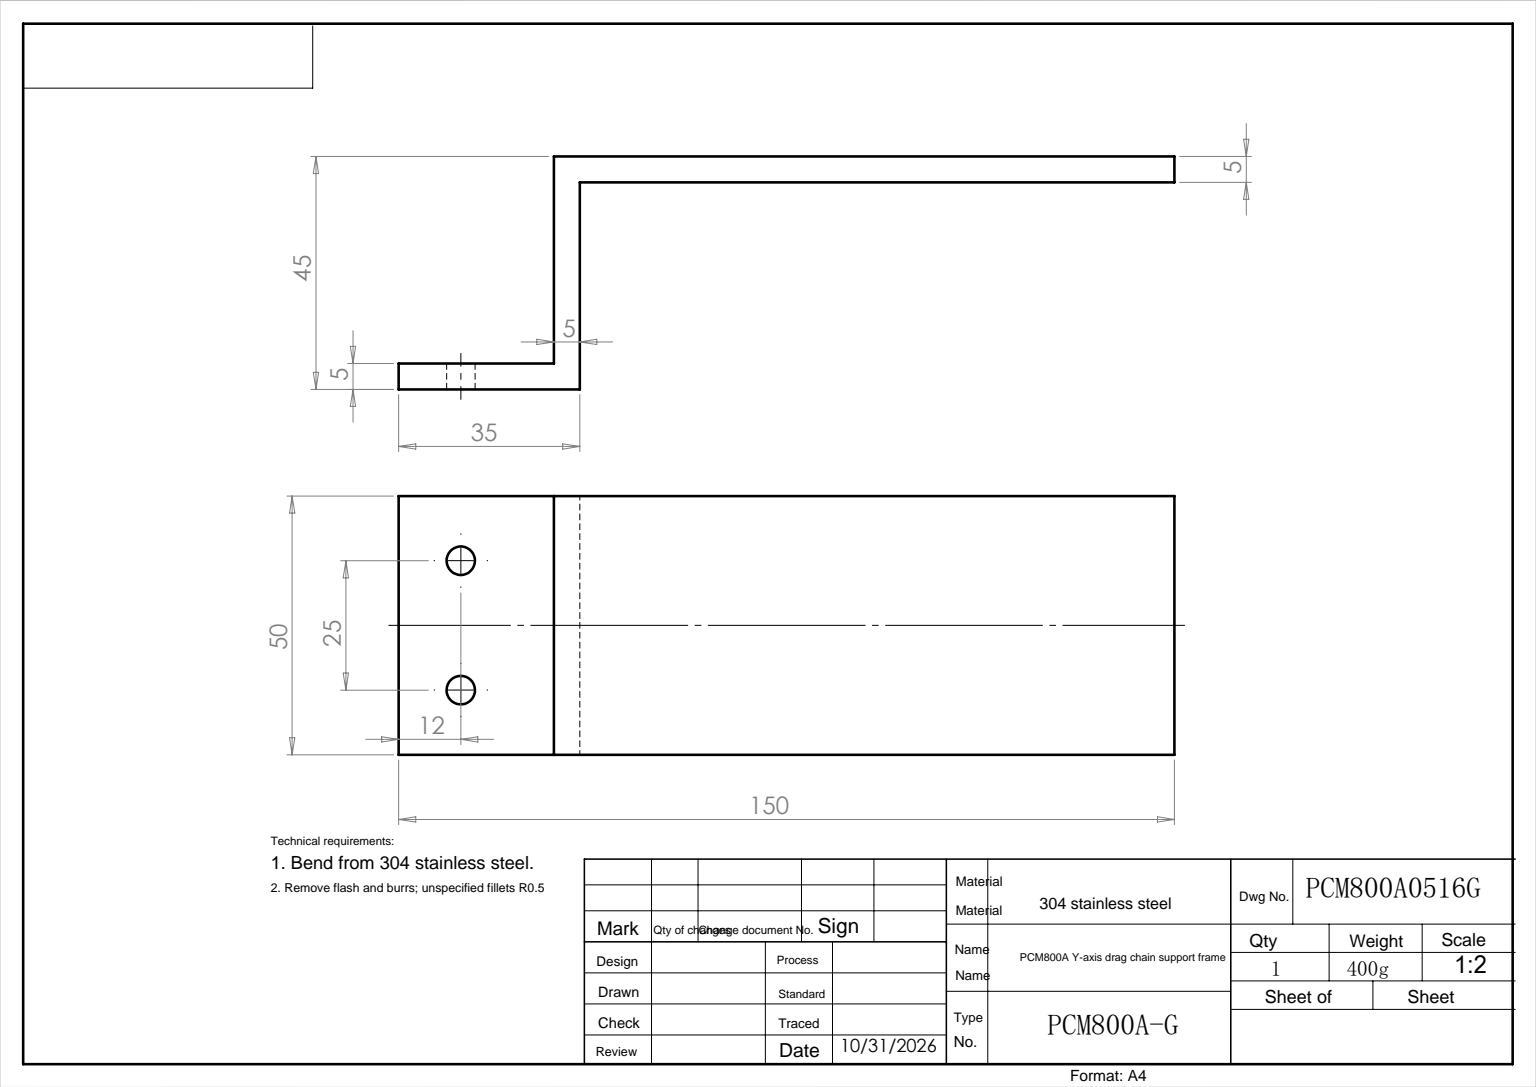
SolidWorks part; units mm, degrees
ref_plane "前视基准面" through (0, 0, 0) normal (0, 0, 1) x (1, 0, 0)
ref_plane "上视基准面" through (0, 0, 0) normal (0, 1, 0) x (1, 0, 0)
ref_plane "右视基准面" through (0, 0, 0) normal (1, 0, 0) x (0, 0, -1)
sketch "草图1" plane through (0, 0, 0) normal (0, 0, 1) x (1, 0, 0)
  line L0 (0, 0) -> (30, 0)
  line L1 (30, 0) -> (30, 40)
  line L2 (30, 40) -> (150, 40)
  dimension "D1" = 40
  dimension "D2" = 30
  dimension "D3" = 120
extrude "拉伸-薄壁1" add sketch "草图1" along normal blind 50 thin
sketch "草图2" plane through (0, 0, 0) normal (0, 1, 0) x (1, 0, 0)
  line L0 (12, -12.5) -> (12, -37.5) construction
  line L2 (0, -25) -> (147.3349, -25) construction
  line L3 (0, -50) -> (0, 0) construction
  circle A0 centre (12, -12.5) radius 2.75
  circle A1 centre (12, -37.5) radius 2.75
  dimension "D1" = 5.5
  dimension "D2" = 12.5
  dimension "D3" = 12
extrude "切除-拉伸1" cut sketch "草图2" against normal blind 10
